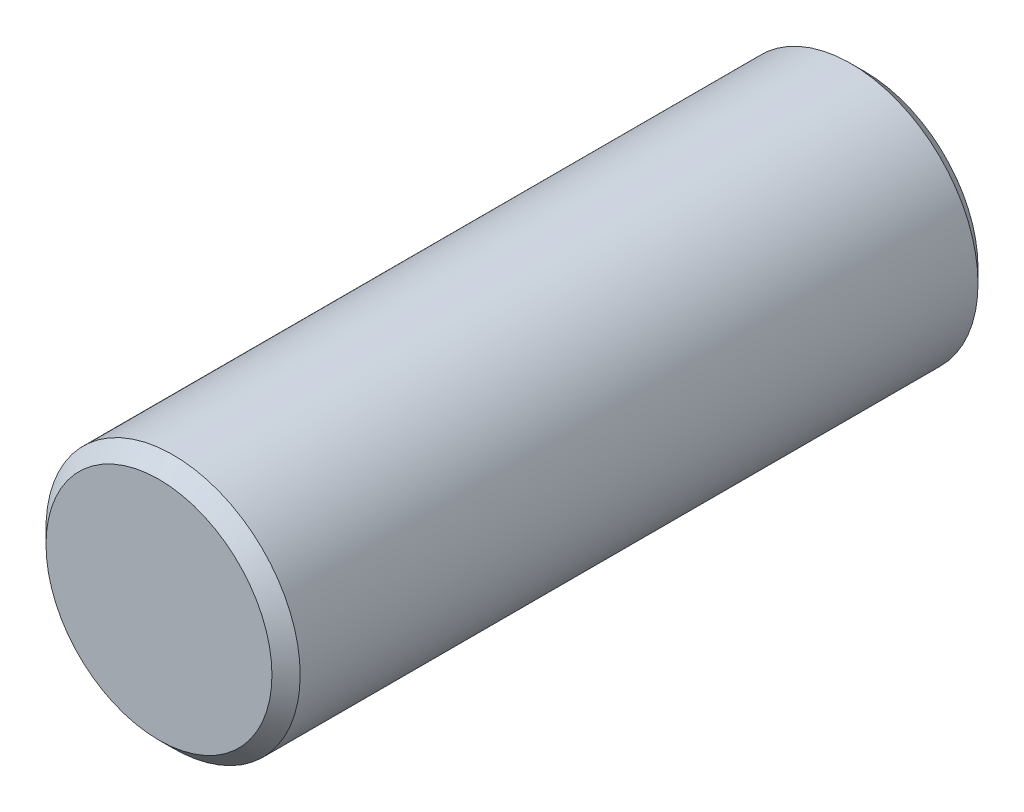
from build123d import *

# Parameters (mm, degrees)
SKETCH1_R           = 9
BOSS_EXTRUDE1_DEPTH = 50
CHAMFER1_SIZE       = 1


with BuildPart() as part:
    # Sketch1 → Boss-Extrude1 (new body)
    with BuildSketch(Plane.XY):
        Circle(SKETCH1_R)
    extrude(amount=BOSS_EXTRUDE1_DEPTH)

    # Chamfer1
    chamfer1_edges = [part.edges().sort_by_distance(p)[0] for p in [
        (-9, 0, 0),
        (-9, 0, 50),
    ]]
    chamfer(chamfer1_edges, length=CHAMFER1_SIZE)


solid = part.part
